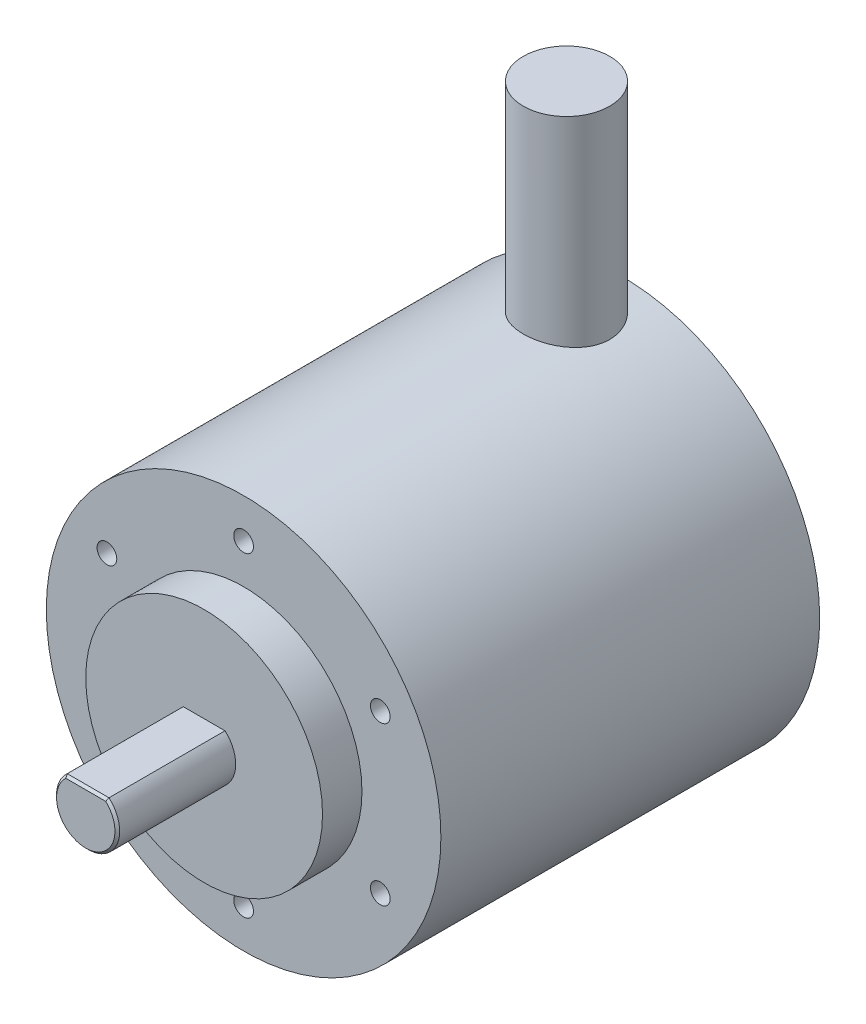
from build123d import *

# Parameters (mm, degrees)
SKETCH1_R           = 25
BOSS_EXTRUDE1_DEPTH = 48
SKETCH2_R           = 15
BOSS_EXTRUDE2_DEPTH = 5
BOSS_EXTRUDE3_DEPTH = 15
CHAMFER1_SIZE       = 0.3
SKETCH4_R           = 5.477956266
BOSS_EXTRUDE4_DEPTH = 50
SKETCH5_R           = 1.25
CUT_EXTRUDE1_DEPTH  = 7


with BuildPart() as part:
    # Sketch1 → Boss-Extrude1 (new body)
    with BuildSketch(Plane.XY):
        Circle(SKETCH1_R)
    extrude(amount=BOSS_EXTRUDE1_DEPTH)

    # Sketch2 → Boss-Extrude2 (add)
    with BuildSketch(Plane.XY.offset(48)):
        Circle(SKETCH2_R)
    extrude(amount=BOSS_EXTRUDE2_DEPTH)

    # Sketch3 → Boss-Extrude3 (add)
    with BuildSketch(Plane.XY.offset(53)):
        with BuildLine():
            Line((-2.645751311, 3), (2.645751311, 3))
            ThreePointArc((2.645751311, 3), (0, -4), (-2.645751311, 3))
        make_face()
    extrude(amount=BOSS_EXTRUDE3_DEPTH)

    # Chamfer1
    chamfer1_edges = [part.edges().sort_by_distance(p)[0] for p in [
        (0, -4, 68),
        (0, 3, 68),
    ]]
    chamfer(chamfer1_edges, length=CHAMFER1_SIZE)

    # Sketch4 → Boss-Extrude4 (add)
    with BuildSketch(Plane(origin=(0, 0, 0), x_dir=(1, 0, 0), z_dir=(0, 1, 0))):
        with Locations(Location((0, -7.083492504, 0), (0, 0, 90))):
            Circle(SKETCH4_R)
    extrude(amount=BOSS_EXTRUDE4_DEPTH)

    # Sketch5 → Cut-Extrude1 (cut)
    with BuildSketch(Plane.XY.offset(48)):
        with Locations((0, 20)):
            Circle(SKETCH5_R)
        with Locations((17.320508076, 10)):
            Circle(SKETCH5_R)
        with Locations((17.320508076, -10)):
            Circle(SKETCH5_R)
        with Locations((0, -20)):
            Circle(SKETCH5_R)
        with Locations((-17.320508076, -10)):
            Circle(SKETCH5_R)
        with Locations((-17.320508076, 10)):
            Circle(SKETCH5_R)
    extrude(amount=-CUT_EXTRUDE1_DEPTH, mode=Mode.SUBTRACT)


solid = part.part
